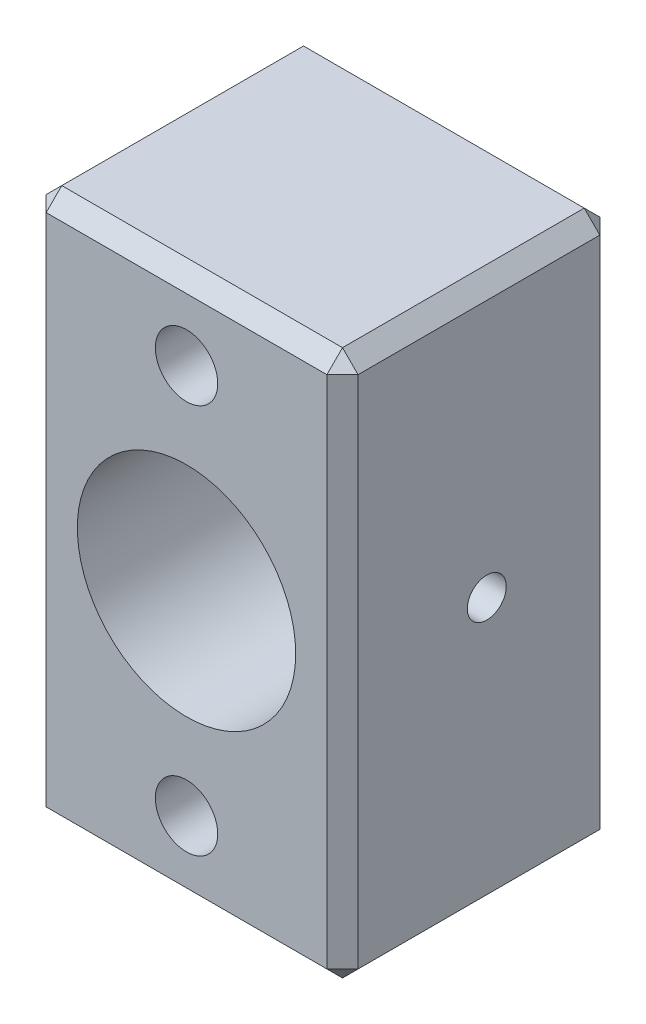
SolidWorks part; units mm, degrees
material "1060 合金"
ref_plane "前视基准面" through (0, 0, 0) normal (0, 0, 1) x (1, 0, 0)
ref_plane "上视基准面" through (0, 0, 0) normal (0, 1, 0) x (1, 0, 0)
ref_plane "右视基准面" through (0, 0, 0) normal (1, 0, 0) x (0, 0, -1)
sketch "草图1" plane through (0, 0, 0) normal (0, 0, 1) x (1, 0, 0)
  line L1 (-20, -35) -> (20, -35)
  line L2 (-20, -35) -> (-20, 35)
  line L3 (-20, 35) -> (20, 35)
  line L4 (20, -35) -> (20, 35)
  line L5 (-20, -35) -> (20, 35) construction
  line L6 (-20, 35) -> (20, -35) construction
  point P0 (0, 0)
  dimension "D1" = 40
  dimension "D2" = 70
extrude "凸台-拉伸1" add sketch "草图1" along normal blind 35
sketch "草图2" plane through (0, 0, 35) normal (0, 0, 1) x (1, 0, 0)
  circle A0 centre (0, 0) radius 14
  dimension "D1" = 28
extrude "切除-拉伸1" cut sketch "草图2" against normal blind 64
sketch "草图4" plane through (0, 0, 35) normal (0, 0, 1) x (1, 0, 0)
  circle A0 centre (0, 25) radius 4
  dimension "D2" = 8
  dimension "D1" = 25
extrude "切除-拉伸3" cut sketch "草图4" against normal blind 59 contours A0
sketch "草图5" plane through (-20, 0, 0) normal (-1, 0, 0) x (0, 0, 1)
  circle A0 centre (16.4988, 0) radius 3.5138
  dimension "D1" = 7.0276
hole_wizard "M6 螺纹孔1" positions "3D草图1" profile "草图6" tap size "M6" standard "GB"
sketch3d "3D草图1"
  point P0 (-20, 0, 16.4988)
sketch "草图6" plane through (-20, 0, 16.4988) normal (0, 1, 0) x (0, 0, 1)
  line L0 (0, 0) -> (0, 6)
  line L1 (0, 6) -> (2.5, 6)
  line L2 (2.5, 6) -> (2.5, 0)
  line L5 (2.5, 0) -> (0, 0)
  line L11 (0, -6.35) -> (0, 107.95) construction
  dimension "通孔螺纹孔钻头直径" = 5
  dimension "通孔螺纹孔钻头深度" = 6
cosmetic thread "孔螺蚊线1" parameters "D2"=6
mirror "镜向2" about plane through (0, 0, 0) normal (0, 1, 0) of "切除-拉伸3"
mirror "镜向3" about plane through (0, 0, 0) normal (1, 0, 0) of "M6 螺纹孔1"
chamfer "倒角1" distance 2 angle 45 12 edges at (-20, -35, 17.5) (0, -35, 35) (20, -35, 17.5) (0, -35, 0) (-20, 35, 17.5) (-20, 0, 35) (0, 35, 35) (20, 0, 35) (-20, 0, 0) (0, 35, 0) (20, 0, 0) (20, 35, 17.5)
